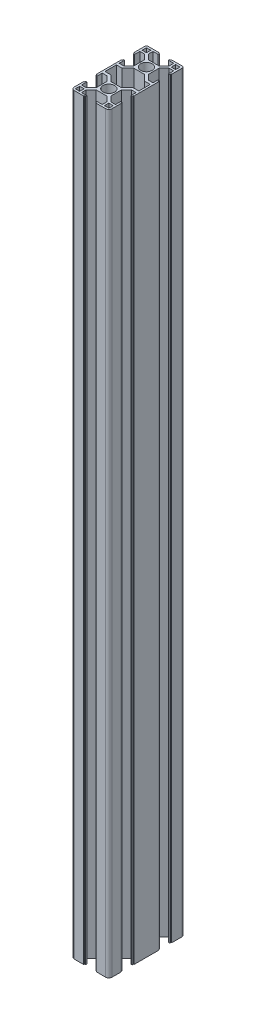
SolidWorks part; units mm, degrees
material "6063 alloy"
ref_plane "Front Plane" through (0, 0, 0) normal (0, 0, 1) x (1, 0, 0)
ref_plane "Top Plane" through (0, 0, 0) normal (0, 1, 0) x (1, 0, 0)
ref_plane "Right Plane" through (0, 0, 0) normal (1, 0, 0) x (0, 0, -1)
sketch "草图1" plane through (0, 0, 0) normal (0, 0, 1) x (1, 0, 0)
  line L0 (0, 0) -> (0, 600)
  dimension "D1" = 600
other "Aluminum profile 30 X 60L X R2.5(1)"
ref_plane "Plane1" through (0, 0, 0) normal (0, 1, 0) x (-1, 0, 0)
sketch "Sketch1" plane through (0, 0, 0) normal (0, 1, 0) x (-1, 0, 0)
  line L0 (-5.1, 15) -> (-5.1, 14.5)
  line L1 (-5.1, 14.5) -> (-4.1, 14.5)
  line L2 (-4.1, 14.5) -> (-4.1, 13.5)
  line L3 (-4.1, 13.5) -> (-8.25, 13.5)
  line L4 (8.9, -10.45) -> (4.25, -5.8)
  line L5 (-15, -24.9) -> (-15, -5.1)
  line L6 (12.5, 15) -> (5.1, 15)
  line L7 (15, 12.5) -> (15, 5.1)
  line L8 (0, 15) -> (0, 0) construction
  line L9 (0, 0) -> (15, 0) construction
  line L10 (-8.25, 13.5) -> (-8.25, 9.8)
  line L11 (-8.25, 9.8) -> (-4.25, 5.8)
  line L12 (-4.25, 5.8) -> (4.25, 5.8)
  line L13 (8.25, 9.8) -> (4.25, 5.8)
  line L14 (8.25, 13.5) -> (8.25, 9.8)
  line L15 (4.1, 13.5) -> (8.25, 13.5)
  line L16 (4.1, 14.5) -> (4.1, 13.5)
  line L17 (5.1, 14.5) -> (4.1, 14.5)
  line L18 (5.1, 15) -> (5.1, 14.5)
  line L19 (-5.1, 15) -> (-12.5, 15)
  line L20 (15, 5.1) -> (14.5, 5.1)
  line L21 (14.5, 5.1) -> (14.5, 4.1)
  line L22 (14.5, 4.1) -> (13.5, 4.1)
  line L23 (13.5, 4.1) -> (13.5, 8.25)
  line L24 (13.5, 8.25) -> (9.8, 8.25)
  line L25 (9.8, 8.25) -> (5.8, 4.25)
  line L26 (5.8, 4.25) -> (5.8, -4.25)
  line L27 (9.8, -8.25) -> (5.8, -4.25)
  line L28 (13.5, -8.25) -> (9.8, -8.25)
  line L29 (13.5, -4.1) -> (13.5, -8.25)
  line L30 (14.5, -4.1) -> (13.5, -4.1)
  line L31 (14.5, -5.1) -> (14.5, -4.1)
  line L32 (15, -5.1) -> (14.5, -5.1)
  line L33 (8.9, -19.55) -> (4.25, -24.2)
  line L34 (-8.9, -19.55) -> (-4.25, -24.2)
  line L35 (-8.9, -10.45) -> (-4.25, -5.8)
  line L36 (-13.5, -10.45) -> (-8.9, -10.45)
  line L37 (-13.5, -19.55) -> (-8.9, -19.55)
  line L38 (-13.5, -10.45) -> (-9.8, -10.45) construction
  line L39 (4.25, -5.8) -> (-4.25, -5.8)
  line L40 (-13.5, -19.55) -> (-9.8, -19.55) construction
  line L41 (-13.5, -10.45) -> (-13.5, -19.55)
  line L42 (13.5, -10.45) -> (13.5, -19.55)
  line L43 (8.9, -10.45) -> (13.5, -10.45)
  line L44 (8.9, -19.55) -> (13.5, -19.55)
  line L45 (-11.625, 11.625) -> (-11.625, 16.245) construction
  line L46 (-15, -5.1) -> (-14.5, -5.1)
  line L47 (-14.5, -5.1) -> (-14.5, -4.1)
  line L48 (-14.5, -4.1) -> (-13.5, -4.1)
  line L49 (-13.5, -4.1) -> (-13.5, -8.25)
  line L50 (-13.5, -8.25) -> (-9.8, -8.25)
  line L51 (-9.8, -8.25) -> (-5.8, -4.25)
  line L52 (-5.8, -4.25) -> (-5.8, 4.25)
  line L53 (-9.8, 8.25) -> (-5.8, 4.25)
  line L54 (-13.5, 8.25) -> (-9.8, 8.25)
  line L55 (-13.5, 4.1) -> (-13.5, 8.25)
  line L56 (-14.5, 4.1) -> (-13.5, 4.1)
  line L57 (-14.5, 5.1) -> (-14.5, 4.1)
  line L58 (-15, 5.1) -> (-14.5, 5.1)
  line L59 (-13.375, 13.375) -> (-9.875, 13.375)
  line L60 (-15, 5.1) -> (-15, 12.5)
  line L61 (15, -5.1) -> (15, -24.9)
  line L62 (-13.375, 13.375) -> (-13.375, 9.875)
  line L63 (-13.375, 9.875) -> (-9.875, 9.875)
  line L64 (-9.875, 13.375) -> (-9.875, 9.875)
  line L65 (-11.625, 11.625) -> (-7.4229, 11.625) construction
  line L66 (-13.5, -45) -> (-5.1, -45)
  line L67 (-15, -43.5) -> (-15, -35.1)
  line L68 (9.875, 13.375) -> (13.375, 13.375)
  line L69 (9.875, 13.375) -> (9.875, 9.875)
  line L70 (9.875, 9.875) -> (13.375, 9.875)
  line L71 (13.375, 13.375) -> (13.375, 9.875)
  line L72 (-4.25, -24.2) -> (4.25, -24.2)
  line L73 (-13.375, -39.875) -> (-9.875, -39.875)
  line L74 (-13.375, -39.875) -> (-13.375, -43.375)
  line L75 (-13.375, -43.375) -> (-9.875, -43.375)
  line L76 (-9.875, -39.875) -> (-9.875, -43.375)
  line L77 (9.875, -39.875) -> (13.375, -39.875)
  line L78 (9.875, -39.875) -> (9.875, -43.375)
  line L79 (9.875, -43.375) -> (13.375, -43.375)
  line L80 (15, -24.9) -> (14.5, -24.9)
  line L81 (14.5, -24.9) -> (14.5, -25.9)
  line L82 (14.5, -25.9) -> (13.5, -25.9)
  line L83 (13.5, -25.9) -> (13.5, -21.75)
  line L84 (13.5, -21.75) -> (9.8, -21.75)
  line L85 (9.8, -21.75) -> (5.8, -25.75)
  line L86 (5.8, -25.75) -> (5.8, -34.25)
  line L87 (9.8, -38.25) -> (5.8, -34.25)
  line L88 (13.5, -38.25) -> (9.8, -38.25)
  line L89 (13.5, -34.1) -> (13.5, -38.25)
  line L90 (14.5, -34.1) -> (13.5, -34.1)
  line L91 (14.5, -35.1) -> (14.5, -34.1)
  line L92 (15, -35.1) -> (14.5, -35.1)
  line L93 (5.1, -45) -> (5.1, -44.5)
  line L94 (5.1, -44.5) -> (4.1, -44.5)
  line L95 (4.1, -44.5) -> (4.1, -43.5)
  line L96 (4.1, -43.5) -> (8.25, -43.5)
  line L97 (8.25, -43.5) -> (8.25, -39.8)
  line L98 (8.25, -39.8) -> (4.25, -35.8)
  line L99 (4.25, -35.8) -> (-4.25, -35.8)
  line L100 (-8.25, -39.8) -> (-4.25, -35.8)
  line L101 (-8.25, -43.5) -> (-8.25, -39.8)
  line L102 (-4.1, -43.5) -> (-8.25, -43.5)
  line L103 (-4.1, -44.5) -> (-4.1, -43.5)
  line L104 (-5.1, -44.5) -> (-4.1, -44.5)
  line L105 (-5.1, -45) -> (-5.1, -44.5)
  line L106 (-15, -35.1) -> (-14.5, -35.1)
  line L107 (-14.5, -35.1) -> (-14.5, -34.1)
  line L108 (-14.5, -34.1) -> (-13.5, -34.1)
  line L109 (-13.5, -34.1) -> (-13.5, -38.25)
  line L110 (-13.5, -38.25) -> (-9.8, -38.25)
  line L111 (-9.8, -38.25) -> (-5.8, -34.25)
  line L112 (-5.8, -34.25) -> (-5.8, -25.75)
  line L113 (-9.8, -21.75) -> (-5.8, -25.75)
  line L114 (-13.5, -21.75) -> (-9.8, -21.75)
  line L115 (-13.5, -25.9) -> (-13.5, -21.75)
  line L116 (-14.5, -25.9) -> (-13.5, -25.9)
  line L117 (-14.5, -24.9) -> (-14.5, -25.9)
  line L118 (-15, -24.9) -> (-14.5, -24.9)
  line L119 (5.1, -45) -> (13.5, -45)
  line L120 (13.375, -39.875) -> (13.375, -43.375)
  line L121 (15, -35.1) -> (15, -43.5)
  line L122 (0, -30) -> (15, -30) construction
  line L125 (5.1, -15) -> (5.1, -14.5) [skipped]
  line L127 (5.1, -14.5) -> (4.1, -14.5) [skipped]
  line L129 (4.1, -14.5) -> (4.1, -13.5) [skipped]
  line L131 (4.1, -13.5) -> (8.25, -13.5) [skipped]
  line L133 (-4.1, -13.5) -> (-8.25, -13.5) [skipped]
  line L135 (-4.1, -14.5) -> (-4.1, -13.5) [skipped]
  line L137 (-5.1, -14.5) -> (-4.1, -14.5) [skipped]
  line L139 (-5.1, -15) -> (-5.1, -14.5) [skipped]
  line L141 (-5.1, -15) -> (-5.1, -15.5) [skipped]
  line L142 (-5.1, -15.5) -> (-4.1, -15.5) [skipped]
  line L143 (-4.1, -15.5) -> (-4.1, -16.5) [skipped]
  line L144 (-4.1, -16.5) -> (-8.25, -16.5) [skipped]
  line L145 (12.5, -15) -> (5.1, -15) [skipped]
  line L146 (4.1, -16.5) -> (8.25, -16.5) [skipped]
  line L147 (4.1, -15.5) -> (4.1, -16.5) [skipped]
  line L148 (5.1, -15.5) -> (4.1, -15.5) [skipped]
  line L149 (5.1, -15) -> (5.1, -15.5) [skipped]
  line L150 (-5.1, -15) -> (-12.5, -15) [skipped]
  line L151 (-15, -24.9) -> (-15, -17.5) [skipped]
  line L152 (15, -17.5) -> (15, -24.9) [skipped]
  line L154 (-8.25, -13.5) -> (-8.25, -9.8) [skipped]
  line L156 (8.25, -13.5) -> (8.25, -9.8) [skipped]
  line L157 (8.25, -16.5) -> (8.25, -20.2) [skipped]
  line L158 (-8.25, -16.5) -> (-8.25, -20.2) [skipped]
  line L160 (-12.5, -14.05) -> (-9.7895, -11.3395) [skipped]
  line L161 (18.444, -10.006) -> (14.8, -13.65) [skipped]
  line L163 (11.9857, -13.5357) -> (9.7894, -11.3394) [skipped]
  line L164 (-15.9344, -12.5156) -> (-14.8, -13.65) [skipped]
  line L165 (9.7894, -15) -> (-9.8, -15) construction
  circle A0 centre (0, 0) radius 4.6
  arc A1 (-15, 12.5) -> (-12.5, 15) centre (-12.5, 12.5) cw
  arc A2 (15, 12.5) -> (12.5, 15) centre (12.5, 12.5) ccw
  arc A3 (15, -43.5) -> (13.5, -45) centre (13.5, -43.5) cw
  arc A4 (-15, -43.5) -> (-13.5, -45) centre (-13.5, -43.5) ccw
  circle A5 centre (0, -30) radius 4.6
  arc A12 (-15, -17.5) -> (-12.5, -15) centre (-12.5, -17.5) cw [skipped]
  arc A13 (15, -17.5) -> (12.5, -15) centre (12.5, -17.5) ccw [skipped]
  point P0 (-10, 0)
  point P1 (10, 0)
  point P2 (0, 20)
  point P4 (0, 0)
  point P5 (0, 0)
  point P6 (-10, 0)
  point P7 (15, 15)
  point P8 (-15, 15)
  point P12 (-15, -15)
  point P13 (15, -15)
  point P15 (0, -10)
  point P16 (10, 0)
  point P36 (-15, 15)
  point P39 (15, 15)
  point P43 (-10, -30)
  point P44 (10, -30)
  point P88 (0, -30)
  point P89 (0, -30)
  point P90 (-10, -30)
  point P91 (10, -30)
  point P102 (15, -45)
  point P120 (-15, -45)
  point P121 (0, 0)
  dimension "D1" = 16.5
  dimension "D2" = 30
  dimension "D3" = 8.2
  dimension "D4" = 10.2
  dimension "D5" = 9.2
  dimension "D6" = 9.2
  dimension "D7" = 2.5
  dimension "D8" = 45
  dimension "D14" = 30
  dimension "D15" = 1.5
  dimension "D9" = 0.5
  dimension "D10" = 1
  dimension "D11" = 8.5
  dimension "D12" = 15
  dimension "D13" = 60
  dimension "D16" = 45
  dimension "D17" = 45
  dimension "D18" = 10.2
  dimension "D19" = 8.2
  dimension "D20" = 2.2
  dimension "D22" = 3.5
  dimension "D21" = 2.2
